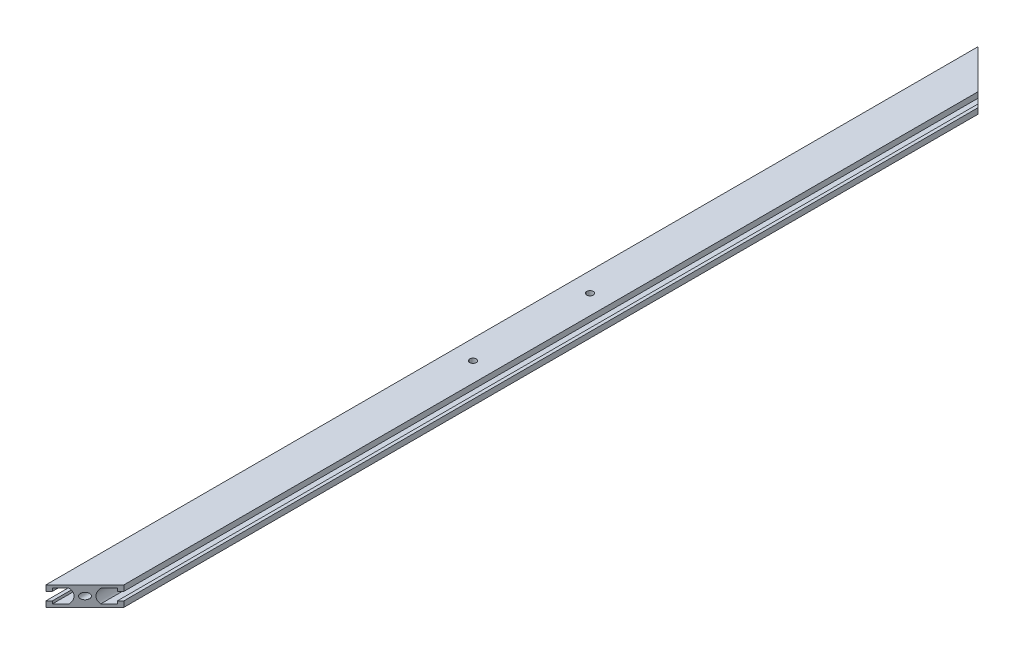
from build123d import *

# Parameters (mm, degrees)
MODEL_R             = 2.5
EXTRUDE_1_DEPTH     = 358.5
CUT_EXTRUDE_1_DEPTH = 2420.679144403
HOLE_WIZARD_M6_1_D  = 5


with BuildPart() as part:
    # Model → 凸台-拉伸1 (new, symmetric)
    with BuildSketch(Plane.XY):
        with BuildLine():
            Line((2390.427059452, 419.756797217), (2392.927059452, 419.756797217))
            Line((2392.927059452, 419.756797217), (2392.927059452, 415.406797217))
            Line((2392.927059452, 415.406797217), (2362.927059452, 415.406797217))
            Line((2362.927059452, 415.406797217), (2362.927059452, 419.756797217))
            Line((2362.927059452, 419.756797217), (2365.427059452, 419.756797217))
            Line((2365.427059452, 419.756797217), (2365.427059452, 417.706797217))
            Line((2365.427059452, 417.706797217), (2371.857059452, 417.706797217))
            ThreePointArc((2371.857059452, 417.706797217), (2373.727059452, 422.906797217), (2371.857059452, 428.106797217))
            Line((2371.857059452, 428.106797217), (2365.427059452, 428.106797217))
            Line((2365.427059452, 428.106797217), (2365.427059452, 426.056797217))
            Line((2365.427059452, 426.056797217), (2362.927059452, 426.056797217))
            Line((2362.927059452, 426.056797217), (2362.927059452, 430.406797217))
            Line((2362.927059452, 430.406797217), (2392.927059452, 430.406797217))
            Line((2392.927059452, 430.406797217), (2392.927059452, 426.056797217))
            Line((2392.927059452, 426.056797217), (2390.427059452, 426.056797217))
            Line((2390.427059452, 426.056797217), (2390.427059452, 428.106797217))
            Line((2390.427059452, 428.106797217), (2383.994799144, 428.106797217))
            ThreePointArc((2383.994799144, 428.106797217), (2382.127059452, 422.906797217), (2383.994799144, 417.706797217))
            Line((2383.994799144, 417.706797217), (2390.427059452, 417.706797217))
            Line((2390.427059452, 417.706797217), (2390.427059452, 419.756797217))
        make_face()
        with Locations((2377.927059452, 422.906797217)):
            Circle(MODEL_R, mode=Mode.SUBTRACT)
    extrude(amount=EXTRUDE_1_DEPTH, both=True)

    # 草图1 → 切除-拉伸1 (cut, through all)
    with BuildSketch(Plane(origin=(0, 430.406797217, 0), x_dir=(1, 0, 0), z_dir=(0, 1, 0))):
        Polygon((2362.927059452, 358.5), (2392.927059452, 328.5), (2392.927059452, 358.5), align=None)
        Polygon((2362.927059452, -358.5), (2392.927059452, -328.5), (2392.927059452, -358.5), align=None)
    extrude(amount=-CUT_EXTRUDE_1_DEPTH, mode=Mode.SUBTRACT)

    # M6 螺纹孔1 (through all)
    with Locations(Plane(origin=(0, 430.406797217, 0), x_dir=(1, 0, 0), z_dir=(0, 1, 0))):
        with Locations((2377.927059452, 45), (2377.927059452, -45)):
            Hole(HOLE_WIZARD_M6_1_D / 2)


solid = part.part
